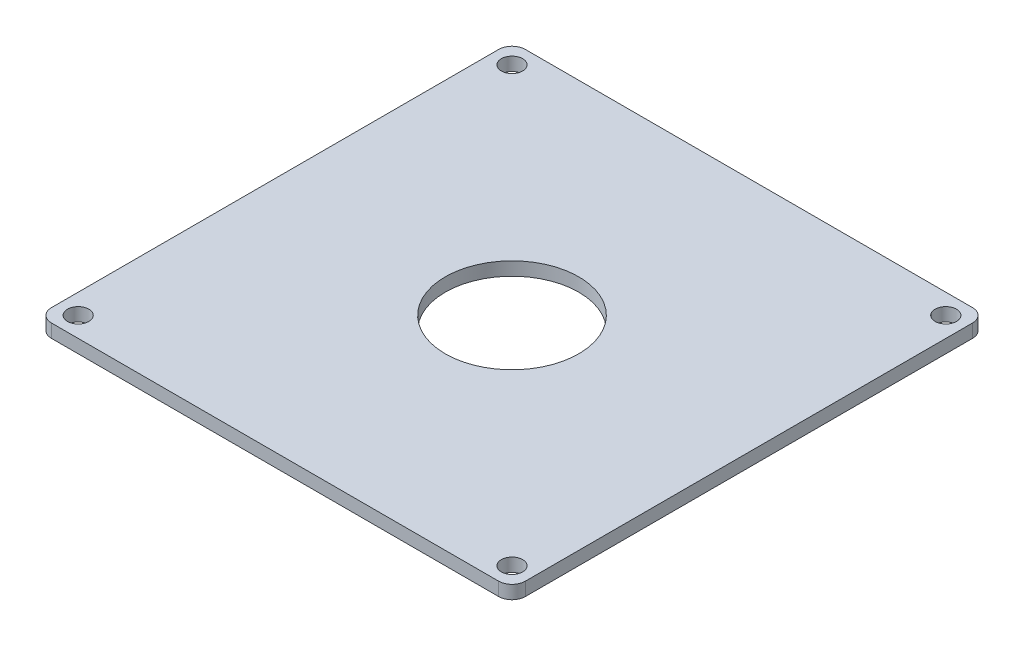
from build123d import *

# Parameters (mm, degrees)
SKETCH1_R           = 1.6
BOSS_EXTRUDE1_DEPTH = 2
SKETCH2_R           = 10
CUT_EXTRUDE1_DEPTH  = 10


with BuildPart() as part:
    # Sketch1 → Boss-Extrude1 (new body)
    with BuildSketch(Plane(origin=(0, 0, 0), x_dir=(1, 0, 0), z_dir=(0, 1, 0))):
        with BuildLine():
            Line((-33.5, -35.5), (33.5, -35.5))
            ThreePointArc((33.5, -35.5), (34.914213562, -34.914213562), (35.5, -33.5))
            Line((35.5, -33.5), (35.5, 33.5))
            ThreePointArc((35.5, 33.5), (34.914213562, 34.914213562), (33.5, 35.5))
            Line((33.5, 35.5), (-33.5, 35.5))
            ThreePointArc((-33.5, 35.5), (-34.914213562, 34.914213562), (-35.5, 33.5))
            Line((-35.5, 33.5), (-35.5, -33.5))
            ThreePointArc((-35.5, -33.5), (-34.914213562, -34.914213562), (-33.5, -35.5))
        make_face()
        with Locations(Location((-32.5, 32.5, 0), (0, 0, 270))):
            Circle(SKETCH1_R, mode=Mode.SUBTRACT)
        with Locations(Location((32.5, 32.5, 0), (0, 0, 270))):
            Circle(SKETCH1_R, mode=Mode.SUBTRACT)
        with Locations(Location((32.5, -32.5, 0), (0, 0, 270))):
            Circle(SKETCH1_R, mode=Mode.SUBTRACT)
        with Locations(Location((-32.5, -32.5, 0), (0, 0, 270))):
            Circle(SKETCH1_R, mode=Mode.SUBTRACT)
    extrude(amount=BOSS_EXTRUDE1_DEPTH)

    # Sketch2 → Cut-Extrude1 (cut)
    with BuildSketch(Plane(origin=(0, 2, 0), x_dir=(1, 0, 0), z_dir=(0, 1, 0))):
        with Locations(Location((0, 0, 0), (0, 0, 270))):
            Circle(SKETCH2_R)
    extrude(amount=-CUT_EXTRUDE1_DEPTH, mode=Mode.SUBTRACT)


solid = part.part
